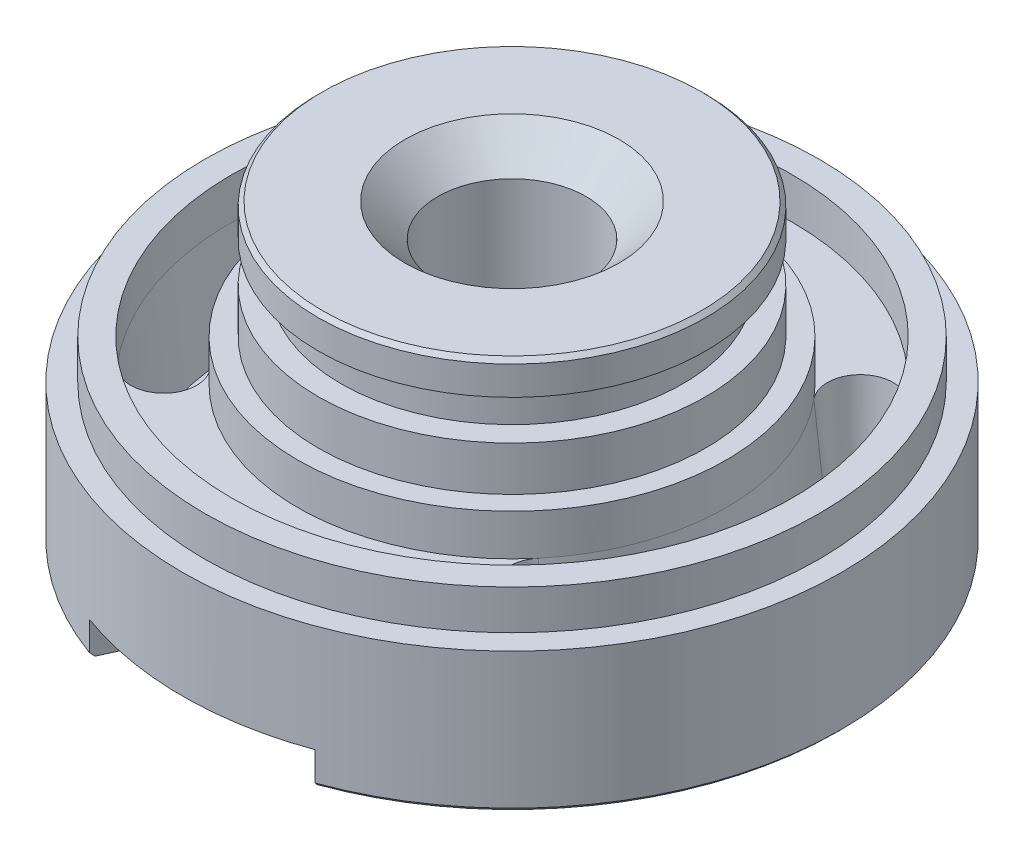
from build123d import *

# Parameters (mm, degrees)
SKETCH1_R                   = 40
BOSS_EXTRUDE1_DEPTH         = 17
SKETCH2_R                   = 37.26
BOSS_EXTRUDE2_DEPTH         = 4.8
SKETCH3_R                   = 23.5
BOSS_EXTRUDE3_DEPTH         = 5.4
SKETCH4_R                   = 20.76
BOSS_EXTRUDE4_DEPTH         = 4.8
SKETCH5_R                   = 23.5
BOSS_EXTRUDE5_DEPTH         = 4
CUT_EXTRUDE1_DEPTH          = 68.052218457
CUT_EXTRUDE1_DEPTH_BACK     = 68.052218457
SKETCH6_R                   = 9
CHAMFER1_SIZE               = 4
CUT_EXTRUDE2_DEPTH          = 61.623757719
CUT_EXTRUDE2_DEPTH_BACK     = 5
SKETCH7_R                   = 34
SKETCH7_R_2                 = 26
CUT_EXTRUDE3_DEPTH          = 4
CUT_EXTRUDE4_DEPTH          = 12.8
CUT_EXTRUDE4_DRAFT          = -5
MIRROR1_COPY_1_DEPTH        = 12.8
MIRROR1_COPY_1_DRAFT        = -5
M4_TAPPED_HOLE1_D           = 3.3
M4_TAPPED_HOLE1_DEPTH       = 11
M4_TAPPED_HOLE1_CSINK_D     = 4.05
M4_TAPPED_HOLE1_CSINK_ANGLE = 90
M4_TAPPED_HOLE1_TIP         = 0.991420021
CUT_EXTRUDE5_DEPTH          = 4
SKETCH15_R                  = 18.5
SKETCH15_R_2                = 14.5
CUT_EXTRUDE6_DEPTH          = 3
CHAMFER2_SIZE               = 0.5


with BuildPart() as part:
    # Sketch1 → Boss-Extrude1 (new body)
    with BuildSketch(Plane(origin=(0, 0, 0), x_dir=(1, 0, 0), z_dir=(0, 1, 0))):
        with Locations(Location((0, 0, 0), (0, 0, 270))):
            Circle(SKETCH1_R)
    extrude(amount=BOSS_EXTRUDE1_DEPTH)

    # Sketch2 → Boss-Extrude2 (add)
    with BuildSketch(Plane(origin=(0, 17, 0), x_dir=(1, 0, 0), z_dir=(0, 1, 0))):
        with Locations(Location((0, 0, 0), (0, 0, 270))):
            Circle(SKETCH2_R)
    extrude(amount=BOSS_EXTRUDE2_DEPTH)

    # Sketch3 → Boss-Extrude3 (add)
    with BuildSketch(Plane(origin=(0, 21.8, 0), x_dir=(1, 0, 0), z_dir=(0, 1, 0))):
        with Locations(Location((0, 0, 0), (0, 0, 270))):
            Circle(SKETCH3_R)
    extrude(amount=BOSS_EXTRUDE3_DEPTH)

    # Sketch4 → Boss-Extrude4 (add)
    with BuildSketch(Plane(origin=(0, 27.2, 0), x_dir=(1, 0, 0), z_dir=(0, 1, 0))):
        with Locations(Location((0, 0, 0), (0, 0, 270))):
            Circle(SKETCH4_R)
    extrude(amount=BOSS_EXTRUDE4_DEPTH)

    # Sketch5 → Boss-Extrude5 (add)
    with BuildSketch(Plane(origin=(0, 32, 0), x_dir=(1, 0, 0), z_dir=(0, 1, 0))):
        with Locations(Location((0, 0, 0), (0, 0, 270))):
            Circle(SKETCH5_R)
    extrude(amount=BOSS_EXTRUDE5_DEPTH)

    # Sketch6 → Cut-Extrude1 (cut, two sides: drawn at the far end of the back side and taken through both)
    with BuildSketch(Plane(origin=(0, 36, 0), x_dir=(1, 0, 0), z_dir=(0, 1, 0)).offset(-CUT_EXTRUDE1_DEPTH_BACK)):
        with Locations(Location((0, 0, 0), (0, 0, 270))):
            Circle(SKETCH6_R)
    extrude(amount=CUT_EXTRUDE1_DEPTH + CUT_EXTRUDE1_DEPTH_BACK, mode=Mode.SUBTRACT)

    # Chamfer1
    chamfer1_edges = [part.edges().sort_by_distance(p)[0] for p in [
        (0, 36, -9),
    ]]
    chamfer(chamfer1_edges, length=CHAMFER1_SIZE)

    # Sketch7 → Cut-Extrude2 (cut, two sides: drawn at the far end of the back side and taken through both)
    with BuildSketch(Plane(origin=(0, 21.8, 0), x_dir=(1, 0, 0), z_dir=(0, 1, 0)).offset(-CUT_EXTRUDE2_DEPTH_BACK)):
        with Locations(Location((0, 0, 0), (0, 0, 270))):
            Circle(SKETCH7_R)
        with Locations(Location((0, 0, 0), (0, 0, 270))):
            Circle(SKETCH7_R_2, mode=Mode.SUBTRACT)
    extrude(amount=CUT_EXTRUDE2_DEPTH + CUT_EXTRUDE2_DEPTH_BACK, mode=Mode.SUBTRACT)

    # Sketch8 → Cut-Extrude3 (cut)
    with BuildSketch(Plane(origin=(0, 0, 0), x_dir=(-1, 0, 0), z_dir=(0, -1, 0))):
        with BuildLine():
            ThreePointArc((25.162362394, -9.790583167), (27, 0), (25.162362394, 9.790583167))
            ThreePointArc((25.162362394, 9.790583167), (28.751993608, 13.771496887), (29.807321036, 8.516079652))
            ThreePointArc((29.807321036, 8.516079652), (31, 0), (29.807321036, -8.516079652))
            ThreePointArc((29.807321036, -8.516079652), (28.751993608, -13.771496887), (25.162362394, -9.790583167))
        make_face()
        with BuildLine():
            ThreePointArc((-25.162362394, 9.790583167), (-28.751993608, 13.771496887), (-29.807321036, 8.516079652))
            ThreePointArc((-29.807321036, 8.516079652), (-31, 0), (-29.807321036, -8.516079652))
            ThreePointArc((-29.807321036, -8.516079652), (-28.751993608, -13.771496887), (-25.162362394, -9.790583167))
            ThreePointArc((-25.162362394, -9.790583167), (-27, 0), (-25.162362394, 9.790583167))
        make_face()
    extrude(amount=-CUT_EXTRUDE3_DEPTH, mode=Mode.SUBTRACT)


with BuildPart() as cut_extrude4_tool:
    # Sketch9 → Cut-Extrude4 (with draft: the straight prism first)
    with BuildSketch(Plane(origin=(0, 16.8, 0), x_dir=(1, 0, 0), z_dir=(0, 1, 0))):
        with BuildLine():
            ThreePointArc((-26.045511066, 21.854778729), (-34, 0), (-26.045511066, -21.854778729))
            ThreePointArc((-26.045511066, -21.854778729), (-20.410182855, -22.347806063), (-19.917155521, -16.712477852))
            ThreePointArc((-19.917155521, -16.712477852), (-26, 0), (-19.917155521, 16.712477852))
            ThreePointArc((-19.917155521, 16.712477852), (-20.410182855, 22.347806063), (-26.045511066, 21.854778729))
        make_face()
    extrude(amount=-CUT_EXTRUDE4_DEPTH)
    # Cut-Extrude4: the draft: its side faces are tilted about the plane it starts from
    cut_extrude4_sides = [cut_extrude4_tool.faces().sort_by_distance(p)[0] for p in [
        (-20.410182855, 10.4, 22.347806063),
        (-26, 10.4, 0),
        (-20.410182855, 10.4, -22.347806063),
        (-34, 10.4, 0),
    ]]
    draft(cut_extrude4_sides, Plane(origin=(0, 16.8, 0), x_dir=(1, 0, 0), z_dir=(0, 1, 0)), CUT_EXTRUDE4_DRAFT)


with BuildPart() as part_1:
    add(part.part)

    # Cut-Extrude4: cut by cut_extrude4_tool
    add(cut_extrude4_tool.part, mode=Mode.SUBTRACT)


with BuildPart() as mirror1_copy_1_tool:
    # Mirror1 copy 1 sketch → Mirror1 copy 1 (with draft: the straight prism first)
    with BuildSketch(Plane(origin=(0, 16.8, 0), x_dir=(-1, 0, 0), z_dir=(0, 1, 0))):
        with BuildLine():
            ThreePointArc((-26.045511066, -21.854778729), (-34, 0), (-26.045511066, 21.854778729))
            ThreePointArc((-26.045511066, 21.854778729), (-20.410182855, 22.347806063), (-19.917155521, 16.712477852))
            ThreePointArc((-19.917155521, 16.712477852), (-26, 0), (-19.917155521, -16.712477852))
            ThreePointArc((-19.917155521, -16.712477852), (-20.410182855, -22.347806063), (-26.045511066, -21.854778729))
        make_face()
    extrude(amount=-MIRROR1_COPY_1_DEPTH)
    # Mirror1 copy 1: the draft: its side faces are tilted about the plane it starts from
    mirror1_copy_1_sides = [mirror1_copy_1_tool.faces().sort_by_distance(p)[0] for p in [
        (20.410182855, 10.4, 22.347806063),
        (26, 10.4, 0),
        (20.410182855, 10.4, -22.347806063),
        (34, 10.4, 0),
    ]]
    draft(mirror1_copy_1_sides, Plane(origin=(0, 16.8, 0), x_dir=(-1, 0, 0), z_dir=(0, 1, 0)), MIRROR1_COPY_1_DRAFT)


with BuildPart() as part_2:
    add(part_1.part)

    # Mirror1 copy 1: cut by mirror1_copy_1_tool
    add(mirror1_copy_1_tool.part, mode=Mode.SUBTRACT)

    # M4 Tapped Hole1
    with Locations(Plane(origin=(0, 0, 0), x_dir=(-1, 0, 0), z_dir=(0, -1, 0))):
        with Locations((36, 0), (-36, 0)):
            CounterSinkHole(M4_TAPPED_HOLE1_D / 2, M4_TAPPED_HOLE1_CSINK_D / 2, depth=M4_TAPPED_HOLE1_DEPTH, counter_sink_angle=M4_TAPPED_HOLE1_CSINK_ANGLE)
            with Locations((0, 0, -(M4_TAPPED_HOLE1_DEPTH + M4_TAPPED_HOLE1_TIP / 2))):  # 118° drill point
                Cone(0, M4_TAPPED_HOLE1_D / 2, M4_TAPPED_HOLE1_TIP, mode=Mode.SUBTRACT)

    # Sketch14 → Cut-Extrude5 (cut)
    with BuildSketch(Plane(origin=(0, 0, 0), x_dir=(-1, 0, 0), z_dir=(0, -1, 0))):
        with BuildLine():
            Line((13.700387767, -37.580571776), (9.977239383, -29.410868278))
            ThreePointArc((9.977239383, -29.410868278), (8.567138417, -27.960848297), (6.557131231, -27.735429148))
            ThreePointArc((6.557131231, -27.735429148), (0, -28.5), (-6.557131231, -27.735429148))
            ThreePointArc((-6.557131231, -27.735429148), (-8.567138417, -27.960848297), (-9.977239383, -29.410868278))
            Line((-9.977239383, -29.410868278), (-13.700387767, -37.580571776))
            ThreePointArc((-13.700387767, -37.580571776), (0, -40), (13.700387767, -37.580571776))
        make_face()
        with BuildLine():
            Line((-13.700387767, 37.580571776), (-9.977239383, 29.410868278))
            ThreePointArc((-9.977239383, 29.410868278), (-8.567138417, 27.960848297), (-6.557131231, 27.735429148))
            ThreePointArc((-6.557131231, 27.735429148), (0, 28.5), (6.557131231, 27.735429148))
            ThreePointArc((6.557131231, 27.735429148), (8.567138417, 27.960848297), (9.977239383, 29.410868278))
            Line((9.977239383, 29.410868278), (13.700387767, 37.580571776))
            ThreePointArc((13.700387767, 37.580571776), (0, 40), (-13.700387767, 37.580571776))
        make_face()
    extrude(amount=-CUT_EXTRUDE5_DEPTH, mode=Mode.SUBTRACT)

    # Sketch15 → Cut-Extrude6 (cut)
    with BuildSketch(Plane(origin=(0, 0, 0), x_dir=(-1, 0, 0), z_dir=(0, -1, 0))):
        with Locations(Location((0, 0, 0), (0, 0, 90))):
            Circle(SKETCH15_R)
        with Locations(Location((0, 0, 0), (0, 0, 90))):
            Circle(SKETCH15_R_2, mode=Mode.SUBTRACT)
    extrude(amount=-CUT_EXTRUDE6_DEPTH, mode=Mode.SUBTRACT)

    # Chamfer2
    chamfer2_edges = [part_2.edges().sort_by_distance(p)[0] for p in [
        (-40, 0, 0),
        (40, 0, 0),
        (0, 36, -23.5),
    ]]
    chamfer(chamfer2_edges, length=CHAMFER2_SIZE)


solid = part_2.part
